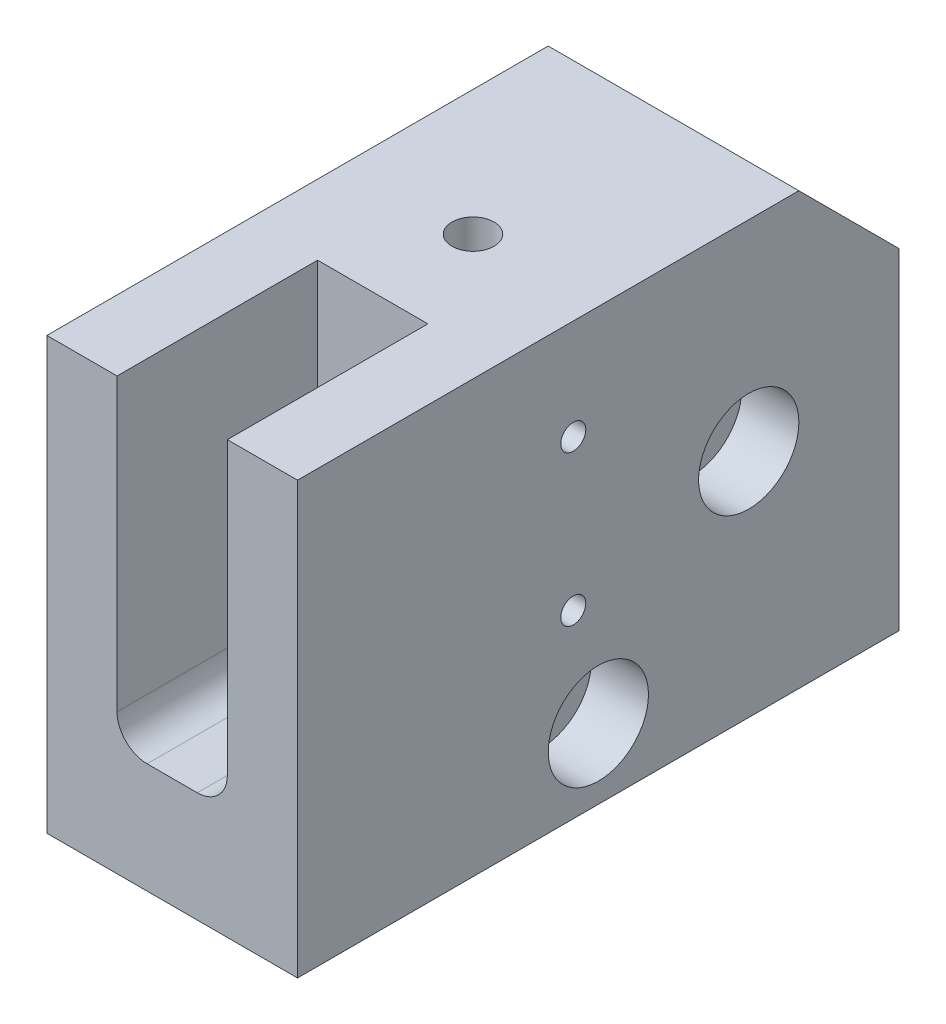
from build123d import *

# Parameters (mm, degrees)
EXTRUDE_THIN1_DEPTH                                  = 30
SKETCH2_W                                            = 60
SKETCH2_H                                            = 12.5
CUT_EXTRUDE1_DEPTH                                   = 92.787798753
SKETCH3_W                                            = 11
SKETCH3_H                                            = 32
CUT_EXTRUDE2_DEPTH                                   = 20
FILLET1_R                                            = 3
SKETCH6_R                                            = 3
CUT_EXTRUDE3_DEPTH                                   = 15
M3_TAPPED_HOLE2_D                                    = 2.5
M3_TAPPED_HOLE2_DEPTH                                = 11.5
M3_TAPPED_HOLE2_TIP                                  = 0.751075774
M5_TAPPED_HOLE1_D                                    = 4.2
M5_TAPPED_HOLE1_DEPTH                                = 12.4
M5_TAPPED_HOLE1_TIP                                  = 1.2618073
CUT_EXTRUDE4_DEPTH                                   = 86.914201472
SKETCH13_W                                           = 35
SKETCH13_H                                           = 12.5
CUT_EXTRUDE6_DEPTH                                   = 1
SKETCH14_W                                           = 10
SKETCH14_H                                           = 59
CUT_EXTRUDE7_DEPTH                                   = 1.5
CHAMFER1_SIZE                                        = 10
SKETCH15_W                                           = 35
SKETCH15_H                                           = 12.5
CUT_EXTRUDE8_DEPTH                                   = 92.137259186
HOLE_SIZE_PER_SOCKET_HEAD_CAP_SCREW_TYPE_D           = 5.5
HOLE_SIZE_PER_SOCKET_HEAD_CAP_SCREW_TYPE_CBORE_D     = 10
HOLE_SIZE_PER_SOCKET_HEAD_CAP_SCREW_TYPE_CBORE_DEPTH = 5.7
SKETCH18_W                                           = 60
SKETCH18_H                                           = 29.5
CUT_EXTRUDE9_DEPTH                                   = 72.589105435
CUT_EXTRUDE10_START                                  = -5.7
SKETCH19_R                                           = 5
CUT_EXTRUDE10_DEPTH                                  = 5.7


with BuildPart() as part:
    # Sketch1 → Extrude-Thin1 (new, symmetric)
    with BuildSketch(Plane.XY):
        Polygon((0, 60), (0, 0), (35, 0), (35, -25), (-25, -25), (-25, 60), align=None)
    extrude(amount=EXTRUDE_THIN1_DEPTH, both=True)

    # Sketch2 → Cut-Extrude1 (cut, through all)
    with BuildSketch(Plane.XY.offset(30)):
        with Locations((5, -18.75)):
            Rectangle(SKETCH2_W, SKETCH2_H)
    extrude(amount=-CUT_EXTRUDE1_DEPTH, mode=Mode.SUBTRACT)

    # Sketch3 → Cut-Extrude2 (cut)
    with BuildSketch(Plane.XY.offset(30)):
        with Locations((-12.5, 44)):
            Rectangle(SKETCH3_W, SKETCH3_H)
    extrude(amount=-CUT_EXTRUDE2_DEPTH, mode=Mode.SUBTRACT)

    # Fillet1
    fillet1_edges = [part.edges().sort_by_distance(p)[0] for p in [
        (-7, 28, 20),
        (-18, 28, 20),
    ]]
    fillet(fillet1_edges, radius=FILLET1_R)

    # Sketch6 → Cut-Extrude3 (cut)
    with BuildSketch(Plane.XY.offset(10)):
        with Locations((-12.5, 50)):
            Circle(SKETCH6_R)
        with Locations((-12.5, 35)):
            Circle(SKETCH6_R)
    extrude(amount=-CUT_EXTRUDE3_DEPTH, mode=Mode.SUBTRACT)

    # M3 Tapped Hole2
    with Locations(Plane(origin=(0, 0, 0), x_dir=(0, 0, -1), z_dir=(1, 0, 0))):
        with Locations((-2.5, 50), (-2.5, 35)):
            Hole(M3_TAPPED_HOLE2_D / 2, depth=M3_TAPPED_HOLE2_DEPTH)
            with Locations((0, 0, -(M3_TAPPED_HOLE2_DEPTH + M3_TAPPED_HOLE2_TIP / 2))):  # 118° drill point
                Cone(0, M3_TAPPED_HOLE2_D / 2, M3_TAPPED_HOLE2_TIP, mode=Mode.SUBTRACT)

    # M5 Tapped Hole1
    with Locations(Plane(origin=(0, 60, 0), x_dir=(-1, 0, 0), z_dir=(0, 1, 0))):
        with Locations((12.5, 0)):
            Hole(M5_TAPPED_HOLE1_D / 2, depth=M5_TAPPED_HOLE1_DEPTH)
            with Locations((0, 0, -(M5_TAPPED_HOLE1_DEPTH + M5_TAPPED_HOLE1_TIP / 2))):  # 118° drill point
                Cone(0, M5_TAPPED_HOLE1_D / 2, M5_TAPPED_HOLE1_TIP, mode=Mode.SUBTRACT)

    # Sketch11 → Cut-Extrude4 (cut, through all)
    with BuildSketch(Plane.XZ.offset(12.5)):
        with BuildLine():
            Line((32.25, -5), (32.25, -25))
            ThreePointArc((32.25, -25), (30, -27.25), (27.75, -25))
            Line((27.75, -25), (27.75, -5))
            ThreePointArc((27.75, -5), (30, -2.75), (32.25, -5))
        make_face()
    extrude(amount=-CUT_EXTRUDE4_DEPTH, mode=Mode.SUBTRACT)

    # Sketch13 → Cut-Extrude6 (cut)
    with BuildSketch(Plane.XY.offset(30)):
        with Locations((17.5, -6.25)):
            Rectangle(SKETCH13_W, SKETCH13_H)
    extrude(amount=-CUT_EXTRUDE6_DEPTH, mode=Mode.SUBTRACT)

    # Sketch14 → Cut-Extrude7 (cut)
    with BuildSketch(Plane(origin=(0, 0, 0), x_dir=(1, 0, 0), z_dir=(0, 1, 0))):
        with Locations((30, 0.5)):
            Rectangle(SKETCH14_W, SKETCH14_H)
    extrude(amount=-CUT_EXTRUDE7_DEPTH, mode=Mode.SUBTRACT)

    # Chamfer1
    chamfer1_edges = [part.edges().sort_by_distance(p)[0] for p in [
        (-12.5, 60, -30),
    ]]
    chamfer(chamfer1_edges, length=CHAMFER1_SIZE)

    # Sketch15 → Cut-Extrude8 (cut, through all)
    with BuildSketch(Plane.XY.offset(29)):
        with Locations((17.5, -6.25)):
            Rectangle(SKETCH15_W, SKETCH15_H)
    extrude(amount=-CUT_EXTRUDE8_DEPTH, mode=Mode.SUBTRACT)

    # Hole Size per Socket Head Cap Screw Type1 (through all)
    with Locations(Plane(origin=(0, 0, 0), x_dir=(0, 0, -1), z_dir=(1, 0, 0))):
        with Locations((0, 24), (15, 40)):
            CounterBoreHole(HOLE_SIZE_PER_SOCKET_HEAD_CAP_SCREW_TYPE_D / 2, HOLE_SIZE_PER_SOCKET_HEAD_CAP_SCREW_TYPE_CBORE_D / 2, HOLE_SIZE_PER_SOCKET_HEAD_CAP_SCREW_TYPE_CBORE_DEPTH)

    # Sketch18 → Cut-Extrude9 (cut, through all)
    with BuildSketch(Plane.ZY.offset(25)):
        with Locations((0, 2.25)):
            Rectangle(SKETCH18_W, SKETCH18_H)
    extrude(amount=-CUT_EXTRUDE9_DEPTH, mode=Mode.SUBTRACT)

    # Sketch19 → Cut-Extrude10 (cut)
    with BuildSketch(Plane.ZY.offset(25).offset(CUT_EXTRUDE10_START)):
        with Locations(Location((-15, 40, 0), (0, 0, 180))):
            Circle(SKETCH19_R)
        with Locations(Location((0, 24, 0), (0, 0, 180))):
            Circle(SKETCH19_R)
    extrude(amount=CUT_EXTRUDE10_DEPTH, mode=Mode.SUBTRACT)


solid = part.part
